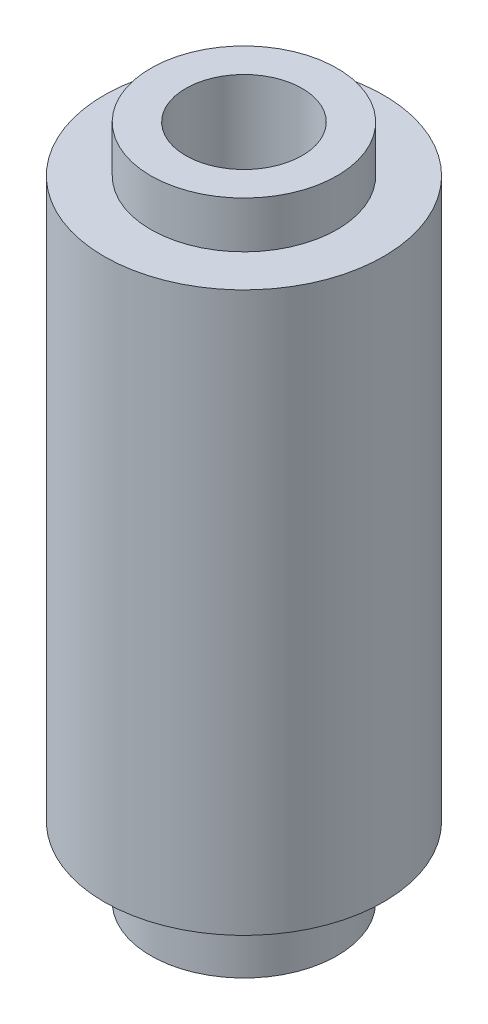
from build123d import *

# Parameters (mm, degrees)
SKETCH_2_R           = 3
BOSS_EXTRUDE_1_DEPTH = 12
SKETCH_3_R           = 2
BOSS_EXTRUDE_2_DEPTH = 1
BOSS_EXTRUDE_START   = 1.5
SKETCH_4_R           = 2
BOSS_EXTRUDE_3_DEPTH = 1.5
SKETCH_5_R           = 1.25
CUT_EXTRUDE_1_DEPTH  = 6
SKETCH_6_R           = 1.5
CUT_EXTRUDE_2_DEPTH  = 2.5
CUT_EXTRUDE_3_DEPTH  = 6


with BuildPart() as part:
    # Sketch 2 → Boss-Extrude 1 (new body)
    with BuildSketch(Plane(origin=(0, 0, 0), x_dir=(1, 0, 0), z_dir=(0, 1, 0))):
        with Locations(Location((0, 0, 0), (0, 0, 270))):
            Circle(SKETCH_2_R)
    extrude(amount=BOSS_EXTRUDE_1_DEPTH)

    # Sketch 3 → Boss-Extrude 2 (add)
    with BuildSketch(Plane(origin=(0, 12, 0), x_dir=(1, 0, 0), z_dir=(0, 1, 0))):
        with Locations(Location((0, 0, 0), (0, 0, 270))):
            Circle(SKETCH_3_R)
    extrude(amount=BOSS_EXTRUDE_2_DEPTH)

    # Sketch 4 → Boss-Extrude 3 (add)
    with BuildSketch(Plane(origin=(0, 0, 0), x_dir=(-1, 0, 0), z_dir=(0, -1, 0)).offset(BOSS_EXTRUDE_START)):
        with Locations(Location((0, 0, 0), (0, 0, 270))):
            Circle(SKETCH_4_R)
    extrude(amount=-BOSS_EXTRUDE_3_DEPTH)

    # Sketch 5 → Cut-Extrude 1 (cut)
    with BuildSketch(Plane(origin=(0, 13, 0), x_dir=(1, 0, 0), z_dir=(0, 1, 0))):
        with Locations(Location((0, 0, 0), (0, 0, 270))):
            Circle(SKETCH_5_R)
    extrude(amount=-CUT_EXTRUDE_1_DEPTH, mode=Mode.SUBTRACT)

    # Sketch 6 → Cut-Extrude 2 (cut)
    with BuildSketch(Plane(origin=(0, 7, 0), x_dir=(1, 0, 0), z_dir=(0, 1, 0))):
        with Locations(Location((0, 0, 0), (0, 0, 270))):
            Circle(SKETCH_6_R)
    extrude(amount=-CUT_EXTRUDE_2_DEPTH, mode=Mode.SUBTRACT)

    # Sketch 7 → Cut-Extrude 3 (cut)
    with BuildSketch(Plane(origin=(0, -1.5, 0), x_dir=(-1, 0, 0), z_dir=(0, -1, 0))):
        Polygon((-0.97407891, 1.14068851), (-1.385866178, -0.57391196), (0.117566508, -1.495385608), (1.458526276, -0.350287172), (0.783852304, 1.27889623), align=None)
    extrude(amount=-CUT_EXTRUDE_3_DEPTH, mode=Mode.SUBTRACT)


solid = part.part
